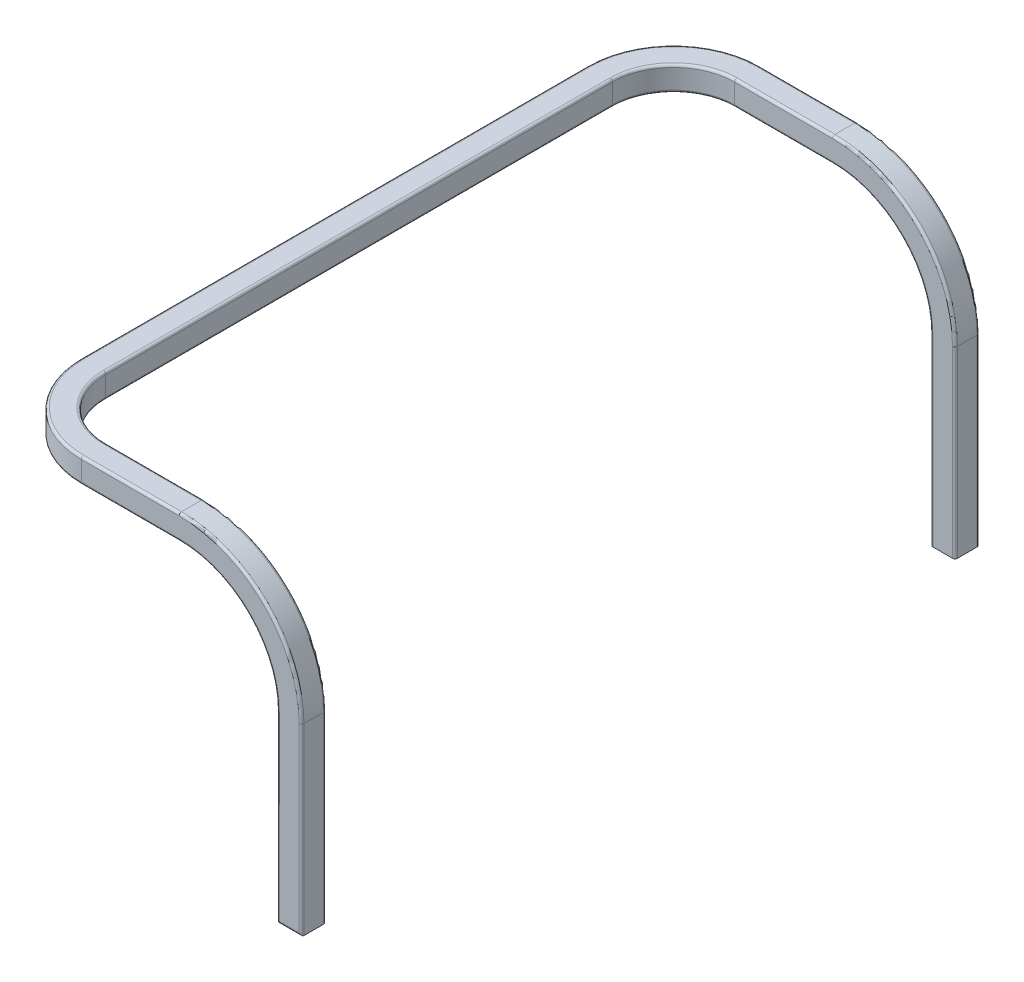
SolidWorks part; units mm, degrees
ref_plane "Front Plane" through (0, 0, 0) normal (0, 0, 1) x (1, 0, 0)
ref_plane "Top Plane" through (0, 0, 0) normal (0, 1, 0) x (1, 0, 0)
ref_plane "Right Plane" through (0, 0, 0) normal (1, 0, 0) x (0, 0, -1)
sketch "Sketch1" plane through (0, 0, 0) normal (0, 0, 1) x (1, 0, 0)
  line L0 (0, 0) -> (0, 150)
  line L1 (-80, 230) -> (-230, 230)
  line L2 (0, 0) -> (20, 0)
  line L3 (20, 0) -> (20, 150)
  line L4 (-80, 250) -> (-230, 250)
  line L5 (-230, 250) -> (-230, 230)
  arc A0 (0, 150) -> (-80, 230) centre (-80, 150) ccw
  arc A1 (20, 150) -> (-80, 250) centre (-80, 150) ccw
  point P11 (20, 250)
  dimension "D5" = 80
  dimension "D6" = 100
  dimension "D1" = 20
  dimension "D3" = 250
  dimension "D4" = 250
  dimension "D7" = 20
extrude "Boss-Extrude1" add sketch "Sketch1" along normal blind 554
sketch "Sketch2" plane through (0, 250, 0) normal (0, 1, 0) x (1, 0, 0)
  line L0 (-80, 0) -> (-230, 0) construction
  line L1 (-210, -534) -> (147.1285, -534)
  line L2 (-210, -534) -> (-210, -20)
  line L3 (-210, -20) -> (147.1285, -20)
  line L4 (147.1285, -534) -> (147.1285, -20)
  line L5 (-80, -554) -> (-230, -554) construction
  line L6 (-230, -554) -> (-230, 0) construction
  dimension "D1" = 20
  dimension "D2" = 20
  dimension "D3" = 20
extrude "Cut-Extrude1" cut sketch "Sketch2" against normal blind 466
fillet "Fillet1" radius 50 2 edges at (-210, 240, 20) (-210, 240, 534)
fillet "Fillet2" radius 70 2 edges at (-230, 240, 0) (-230, 240, 554)
fillet "Fillet3" radius 2 38 edges at (20, 75, 20) (-9.2893, 220.7107, 20) (-120, 250, 20) (-195.3553, 250, 34.6447) (-210, 250, 277) (-195.3553, 250, 519.3553) (0, 75, 20) (-23.4315, 206.5685, 20) (-120, 230, 20) (-195.3553, 230, 34.6447) (-210, 230, 277) (-195.3553, 230, 519.3553) (0, 75, 0) (-23.4315, 206.5685, 0) (-120, 230, 0) (-209.4975, 230, 20.5025) (-230, 230, 277) (-209.4975, 230, 533.4975) (20, 75, 0) (-9.2893, 220.7107, 0) (-120, 250, 0) (-209.4975, 250, 20.5025) (-230, 250, 277) (-209.4975, 250, 533.4975) (-23.4315, 206.5685, 534) (0, 75, 534) (10, 0, 534) (20, 75, 534) (-9.2893, 220.7107, 534) (-120, 250, 534) (-120, 230, 534) (-9.2893, 220.7107, 554) (20, 75, 554) (10, 0, 554) (0, 75, 554) (-23.4315, 206.5685, 554) (-120, 230, 554) (-120, 250, 554)
